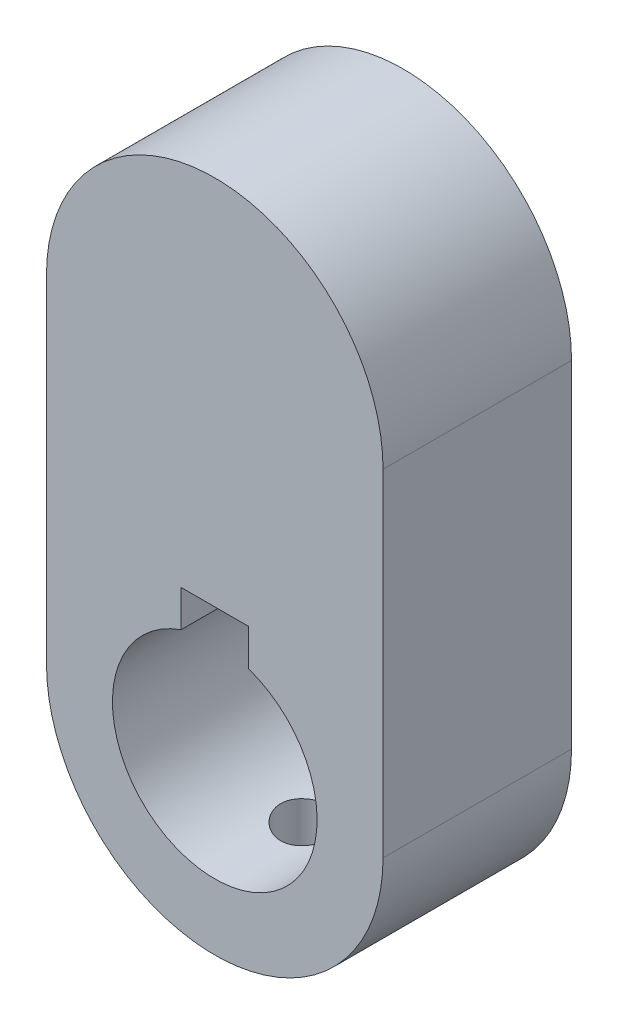
from build123d import *

# Parameters (mm, degrees)
BOSS_EXTRUDE1_DEPTH = 14
SKETCH3_W           = 2.1
SKETCH3_H           = 12.5


with BuildPart() as part:
    # Sketch1 → Boss-Extrude1 (new body)
    with BuildSketch(Plane.XY):
        with BuildLine():
            Line((-12.5, 25), (-12.5, 0))
            ThreePointArc((-12.5, 0), (0, -12.5), (12.5, 0))
            Line((12.5, 0), (12.5, 25))
            ThreePointArc((12.5, 25), (0, 37.5), (-12.5, 25))
        make_face()
        with BuildLine():
            Line((2.5, 9.9), (2.5, 7.177046746))
            ThreePointArc((2.5, 7.177046746), (6.195159401, 4.402272141), (7.6, 0))
            ThreePointArc((7.6, 0), (-4.402272141, -6.195159401), (-2.5, 7.177046746))
            Line((-2.5, 7.177046746), (-2.5, 9.9))
            Line((-2.5, 9.9), (2.5, 9.9))
        make_face(mode=Mode.SUBTRACT)
    extrude(amount=BOSS_EXTRUDE1_DEPTH)

    # Sketch3 → M5 Tapped Hole1 (revolve, cut)
    with BuildSketch(Plane(origin=(0, 0, 7), x_dir=(0, 0, 1), z_dir=(1, 0, 0))):
        with Locations((1.05, 6.25)):
            Rectangle(SKETCH3_W, SKETCH3_H)
    revolve(axis=Axis((0, 6.35, 7), (0, -1, 0)), mode=Mode.SUBTRACT)


solid = part.part
